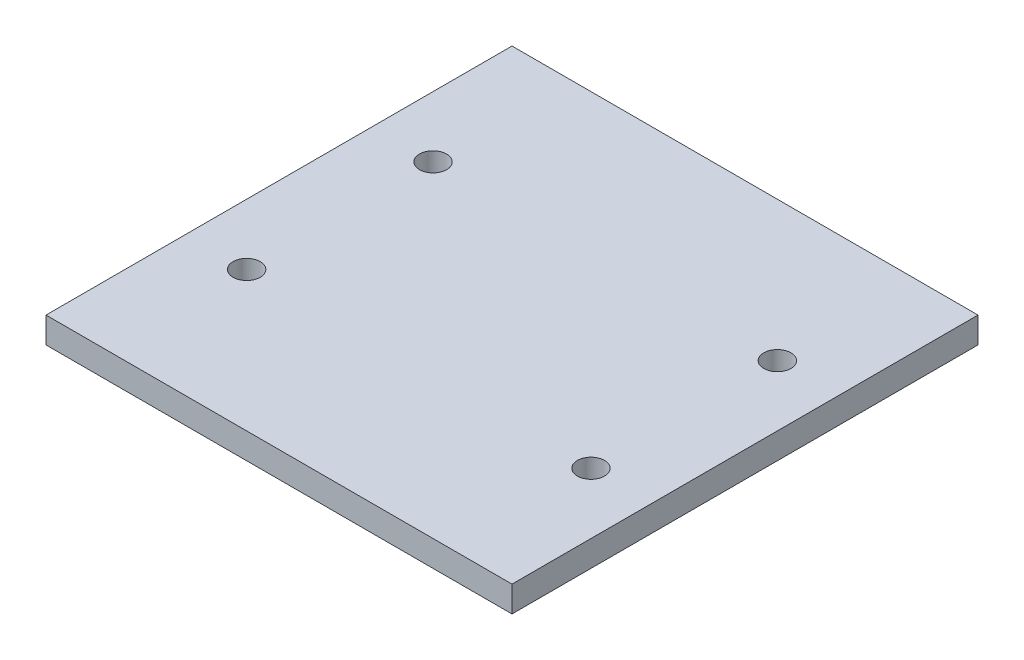
from build123d import *

# Parameters (mm, degrees)
SKETCH1_W            = 360
SKETCH1_H            = 360
EXTRUDE1_DEPTH       = 10
M24_TAPPED_HOLE1_D   = 21
LPATTERN2_COUNT      = 2
LPATTERN2_PITCH      = 144
LPATTERN2_COUNT_DIR2 = 2
LPATTERN2_PITCH_DIR2 = 266


with BuildPart() as part:
    # Sketch1 → Extrude1 (new, symmetric)
    with BuildSketch(Plane(origin=(0, 0, 0), x_dir=(1, 0, 0), z_dir=(0, 1, 0))):
        Rectangle(SKETCH1_W, SKETCH1_H)
    extrude(amount=EXTRUDE1_DEPTH, both=True)

    # M24 Tapped Hole1 (through all)
    with Locations(Plane(origin=(0, 10, 0), x_dir=(-1, 0, 0), z_dir=(0, 1, 0))):
        with Locations((133, -72)):
            m24_tapped_hole1 = Hole(M24_TAPPED_HOLE1_D / 2)

    # LPattern2: M24 Tapped Hole1 2 × 2
    with Locations(*[(j * LPATTERN2_PITCH_DIR2, 0, i * LPATTERN2_PITCH) for i in range(LPATTERN2_COUNT) for j in range(LPATTERN2_COUNT_DIR2) if (i, j) != (0, 0)]):
        add(m24_tapped_hole1, mode=Mode.SUBTRACT)


solid = part.part
